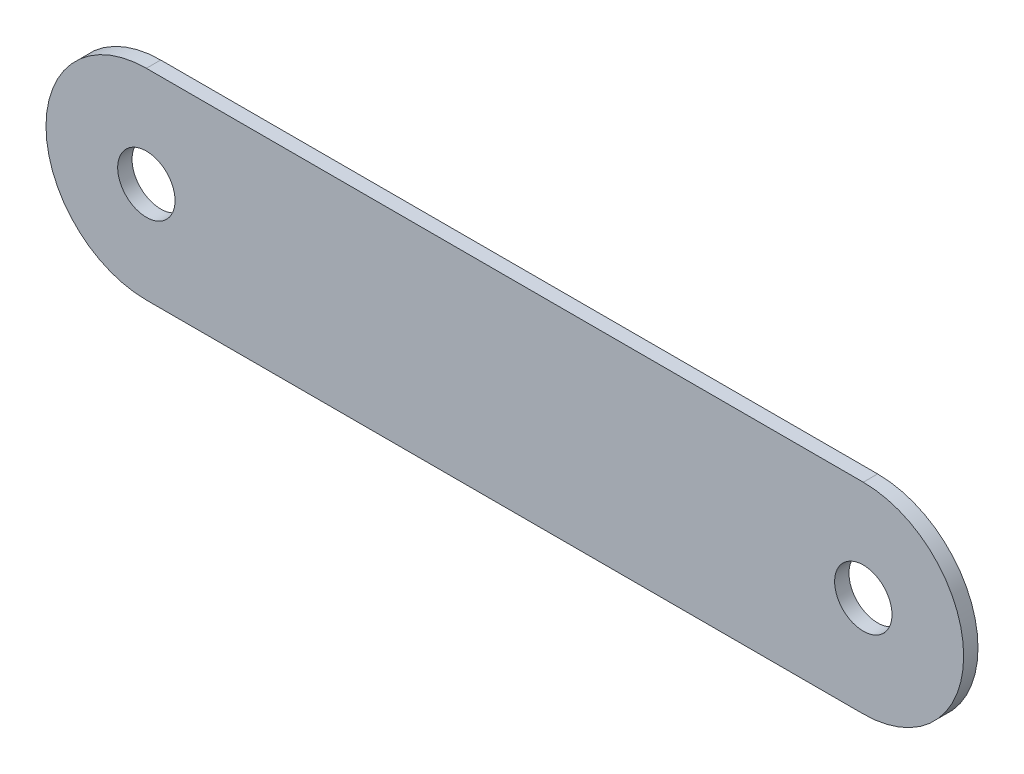
from build123d import *

# Parameters (mm, degrees)
SKETCH1_R           = 2
BOSS_EXTRUDE1_DEPTH = 1


with BuildPart() as part:
    # Sketch1 → Boss-Extrude1 (new body)
    with BuildSketch(Plane.XY):
        with BuildLine():
            Line((-33.139059677, 7), (16.860940323, 7))
            ThreePointArc((16.860940323, 7), (23.860940323, 0), (16.860940323, -7))
            Line((16.860940323, -7), (-33.139059677, -7))
            ThreePointArc((-33.139059677, -7), (-40.139059677, 0), (-33.139059677, 7))
        make_face()
        with Locations((-33.139059677, 0)):
            Circle(SKETCH1_R, mode=Mode.SUBTRACT)
        with Locations((16.860940323, 0)):
            Circle(SKETCH1_R, mode=Mode.SUBTRACT)
    extrude(amount=BOSS_EXTRUDE1_DEPTH)


solid = part.part
